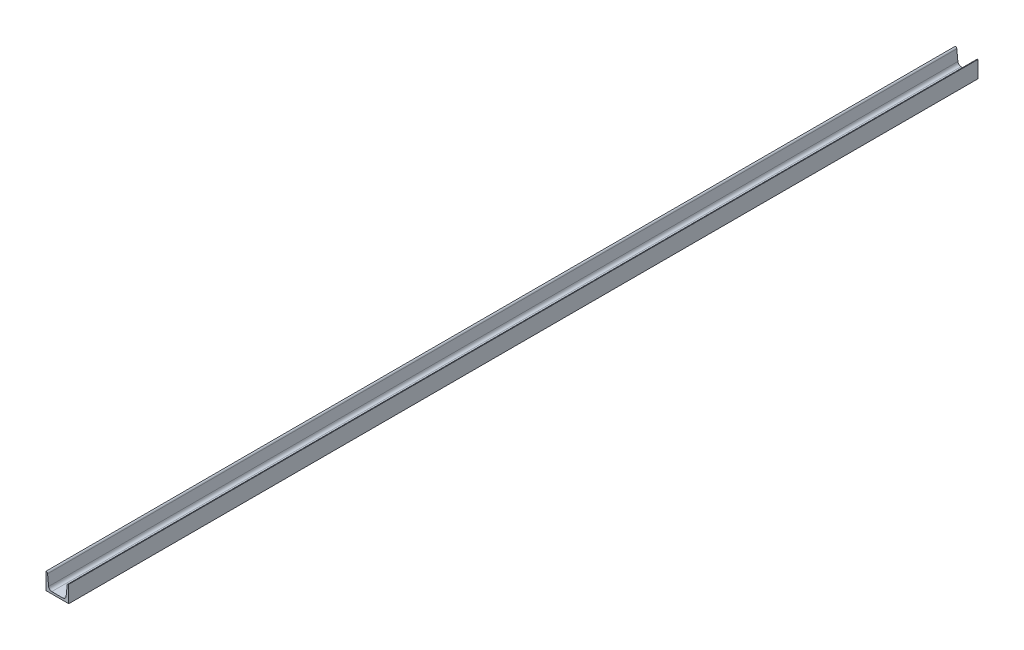
SolidWorks part; units mm, degrees
material "普通碳钢"
ref_plane "Front Plane" through (0, 0, 0) normal (0, 0, 1) x (1, 0, 0)
ref_plane "Top Plane" through (0, 0, 0) normal (0, 1, 0) x (1, 0, 0)
ref_plane "Right Plane" through (0, 0, 0) normal (1, 0, 0) x (0, 0, -1)
sketch "Sketch1" plane through (0, 0, 0) normal (0, 0, 1) x (1, 0, 0)
  line L0 (-25, 0) -> (25, 0)
  line L1 (25, 0) -> (25, 37)
  line L2 (-25, 0) -> (-25, 37)
  line L3 (-21.55, 33.8478) -> (-19.25, 10.8048)
  line L4 (-12.2846, 4.5) -> (12.2846, 4.5)
  line L5 (21.55, 33.8478) -> (19.25, 10.8048)
  line L6 (20.4, 22.3263) -> (20.4, 0) construction
  line L7 (0, 0) -> (0, 29.3406) construction
  arc A0 (21.55, 33.8478) -> (25, 37) centre (25.0327, 33.5002) cw
  arc A1 (12.2846, 4.5) -> (19.25, 10.8048) centre (12.2846, 11.5) ccw
  arc A2 (-21.55, 33.8478) -> (-25, 37) centre (-25.0327, 33.5002) ccw
  arc A3 (-12.2846, 4.5) -> (-19.25, 10.8048) centre (-12.2846, 11.5) cw
  point P4 (0, 0)
  point P21 (0, 4.5)
  dimension "D4" = 7
  dimension "D5" = 3.5
  dimension "D1" = 50
  dimension "D2" = 37
  dimension "D3" = 4.5
  dimension "D6" = 5.7
  dimension "D7" = 4.6
extrude "Extrude1" add sketch "Sketch1" along normal mid plane 2000
